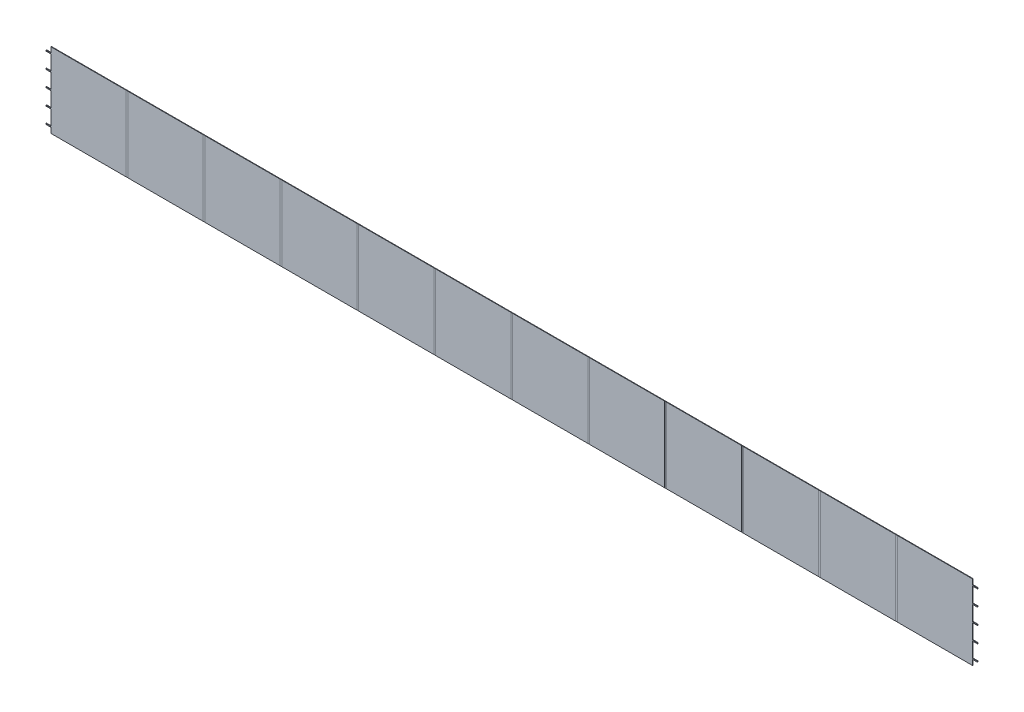
SolidWorks part; units mm, degrees
ref_plane "前视" through (0, 0, 0) normal (0, 0, 1) x (1, 0, 0)
ref_plane "上视" through (0, 0, 0) normal (0, 1, 0) x (1, 0, 0)
ref_plane "右视" through (0, 0, 0) normal (1, 0, 0) x (0, 0, -1)
sketch "草图1" plane through (0, 0, 0) normal (0, 0, 1) x (1, 0, 0)
  line L1 (0, 0) -> (1916, 0)
  line L2 (0, 0) -> (0, -156)
  line L3 (0, -156) -> (1916, -156)
  line L4 (1916, 0) -> (1916, -156)
  dimension "D1" = 156
  dimension "D2" = 1916
extrude "凸台-拉伸1" add sketch "草图1" along normal blind 1
sketch "草图2" plane through (0, 0, 1) normal (0, 0, 1) x (1, 0, 0)
  line L1 (0, 0) -> (156, 0)
  line L2 (0, 0) -> (0, -156)
  line L3 (0, -156) -> (156, -156)
  line L4 (156, 0) -> (156, -156)
  line L5 (0, 0) -> (0, -156) construction
  line L6 (160, -156) -> (316, -156)
  line L7 (160, 0) -> (316, 0)
  line L8 (316, 0) -> (316, -156)
  line L9 (160, 0) -> (160, -156)
  line L10 (320, -156) -> (476, -156)
  line L11 (320, 0) -> (476, 0)
  line L12 (476, 0) -> (476, -156)
  line L13 (320, 0) -> (320, -156)
  line L14 (480, -156) -> (636, -156)
  line L15 (480, 0) -> (636, 0)
  line L16 (636, 0) -> (636, -156)
  line L17 (480, 0) -> (480, -156)
  line L18 (640, -156) -> (796, -156)
  line L19 (640, 0) -> (796, 0)
  line L20 (796, 0) -> (796, -156)
  line L21 (640, 0) -> (640, -156)
  line L22 (800, -156) -> (956, -156)
  line L23 (800, 0) -> (956, 0)
  line L24 (956, 0) -> (956, -156)
  line L25 (800, 0) -> (800, -156)
  line L26 (960, -156) -> (1116, -156)
  line L27 (960, 0) -> (1116, 0)
  line L28 (1116, 0) -> (1116, -156)
  line L29 (960, 0) -> (960, -156)
  line L30 (1120, -156) -> (1276, -156)
  line L31 (1120, 0) -> (1276, 0)
  line L32 (1276, 0) -> (1276, -156)
  line L33 (1120, 0) -> (1120, -156)
  line L34 (1280, -156) -> (1436, -156)
  line L35 (1280, 0) -> (1436, 0)
  line L36 (1436, 0) -> (1436, -156)
  line L37 (1280, 0) -> (1280, -156)
  line L38 (1440, -156) -> (1596, -156)
  line L39 (1440, 0) -> (1596, 0)
  line L40 (1596, 0) -> (1596, -156)
  line L41 (1440, 0) -> (1440, -156)
  line L42 (1600, -156) -> (1756, -156)
  line L43 (1600, 0) -> (1756, 0)
  line L44 (1756, 0) -> (1756, -156)
  line L45 (1600, 0) -> (1600, -156)
  line L46 (1760, -156) -> (1916, -156)
  line L47 (1760, 0) -> (1916, 0)
  line L48 (1916, 0) -> (1916, -156)
  line L49 (1760, 0) -> (1760, -156)
  dimension "D1" = 156
  dimension "D4" = 4
  dimension "D3" = 12
extrude "凸台-拉伸2" add sketch "草图2" along normal blind 0.1
ref_plane "基准面1" through (958, 0, 0) normal (-1, 0, 0) x (0, 0, 1)
sketch "草图3" plane through (0, 0, 1.1) normal (0, 0, 1) x (1, 0, 0)
  line L0 (0, 0) -> (0, -156) construction
  line L1 (-10, -11) -> (10, -11)
  line L2 (-10, -11) -> (-10, -13)
  line L3 (-10, -13) -> (10, -13)
  line L4 (10, -11) -> (10, -13)
  line L5 (-10, -44) -> (10, -44)
  line L6 (-10, -46) -> (10, -46)
  line L7 (10, -44) -> (10, -46)
  line L8 (-10, -44) -> (-10, -46)
  line L9 (-10, -77) -> (10, -77)
  line L10 (-10, -79) -> (10, -79)
  line L11 (10, -77) -> (10, -79)
  line L12 (-10, -77) -> (-10, -79)
  line L13 (-10, -110) -> (10, -110)
  line L14 (-10, -112) -> (10, -112)
  line L15 (10, -110) -> (10, -112)
  line L16 (-10, -110) -> (-10, -112)
  line L17 (-10, -143) -> (10, -143)
  line L18 (-10, -145) -> (10, -145)
  line L19 (10, -143) -> (10, -145)
  line L20 (-10, -143) -> (-10, -145)
  line L21 (156, 0) -> (0, 0) construction
  dimension "D1" = 2
  dimension "D2" = 10
  dimension "D3" = 10
  dimension "D5" = 11
  dimension "D4" = 5
extrude "凸台-拉伸3" add sketch "草图3" against normal blind 1.1
mirror "镜向1" about plane through (958, 0, 0) normal (-1, 0, 0) of "凸台-拉伸3"
